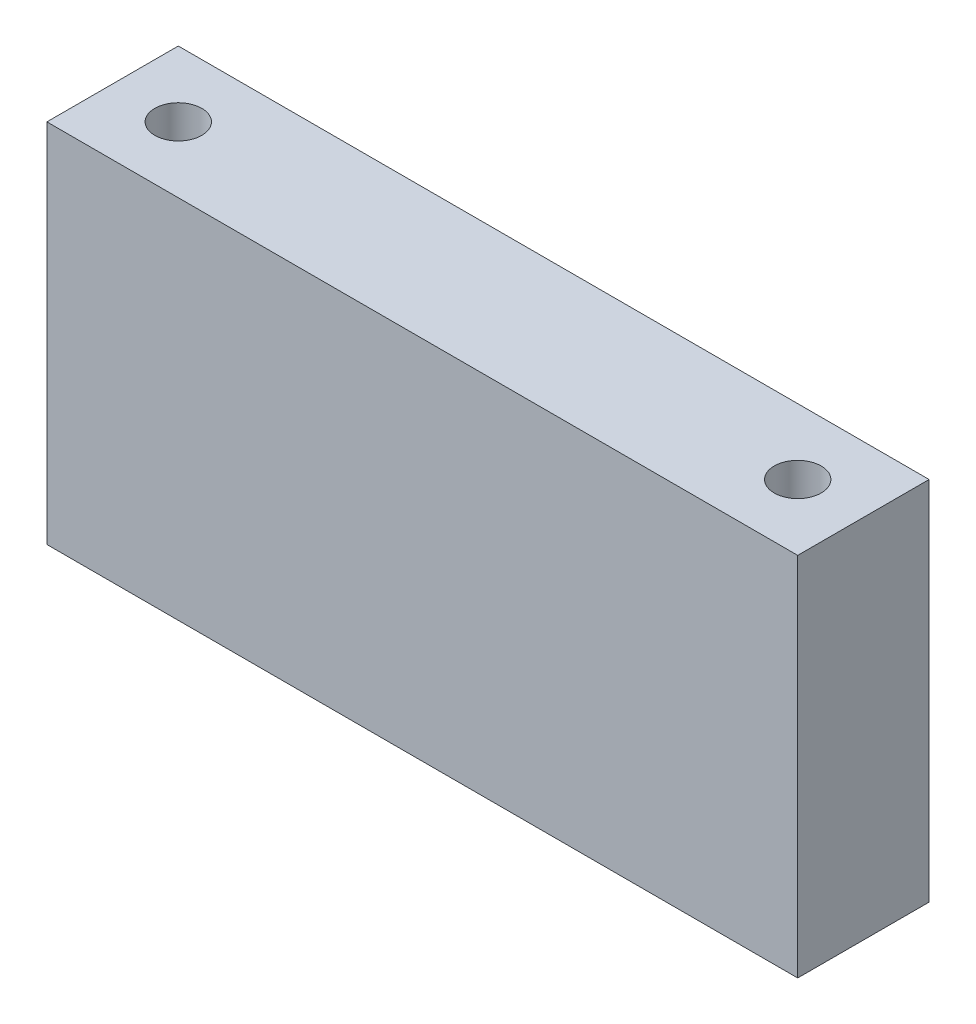
SolidWorks part; units mm, degrees
ref_plane "前视" through (0, 0, 0) normal (0, 0, 1) x (1, 0, 0)
ref_plane "上视" through (0, 0, 0) normal (0, 1, 0) x (1, 0, 0)
ref_plane "右视" through (0, 0, 0) normal (1, 0, 0) x (0, 0, -1)
sketch "草图1" plane through (0, 0, 0) normal (0, 0, 1) x (1, 0, 0)
  line L1 (-40, 19.5) -> (40, 19.5)
  line L2 (-40, 19.5) -> (-40, -19.5)
  line L3 (-40, -19.5) -> (40, -19.5)
  line L4 (40, 19.5) -> (40, -19.5)
  line L5 (-40, 19.5) -> (40, -19.5) construction
  line L6 (-40, -19.5) -> (40, 19.5) construction
  point P0 (0, 0)
  dimension "D1" = 80
  dimension "D2" = 39
extrude "凸台-拉伸1" add sketch "草图1" along normal blind 14
hole_wizard "M6 螺纹孔1" positions "草图3" profile "草图2" tap size "M6" standard "GB"
sketch "草图3" plane through (0, -19.5, 0) normal (0, -1, 0) x (-1, 0, 0)
  point P0 (-21, -7)
  point P3 (21, -7)
sketch "草图2" plane through (21, -19.5, 7) normal (1, 0, 0) x (0, 0, -1)
  line L0 (0, 0) -> (0, 18.5022)
  line L1 (0, 18.5022) -> (2.5, 17)
  line L2 (2.5, 17) -> (2.5, 0)
  line L5 (2.5, 0) -> (0, 0)
  line L10 (0, 18.5022) -> (-2.5, 17) construction
  line L11 (0, -6.35) -> (0, 107.95) construction
  dimension "螺纹孔钻头直径" = 5
  dimension "螺纹孔钻头深度" = 17
  dimension "导头角度" = 118
cosmetic thread "孔螺蚊线1"
cosmetic thread "孔螺蚊线2"
hole_wizard "M6 螺纹孔2" positions "草图5" profile "草图4" tap size "M6" standard "GB"
sketch "草图5" plane through (0, 19.5, 0) normal (0, 1, 0) x (1, 0, 0)
  point P0 (-33, -7)
  point P2 (33, -7)
sketch "草图4" plane through (-33, 19.5, 7) normal (1, 0, 0) x (0, 0, 1)
  line L0 (0, 0) -> (0, 18.5022)
  line L1 (0, 18.5022) -> (2.5, 17)
  line L2 (2.5, 17) -> (2.5, 0)
  line L5 (2.5, 0) -> (0, 0)
  line L10 (0, 18.5022) -> (-2.5, 17) construction
  line L11 (0, -6.35) -> (0, 107.95) construction
  dimension "螺纹孔钻头直径" = 5
  dimension "螺纹孔钻头深度" = 17
  dimension "导头角度" = 118
cosmetic thread "孔螺蚊线3"
cosmetic thread "孔螺蚊线4"
